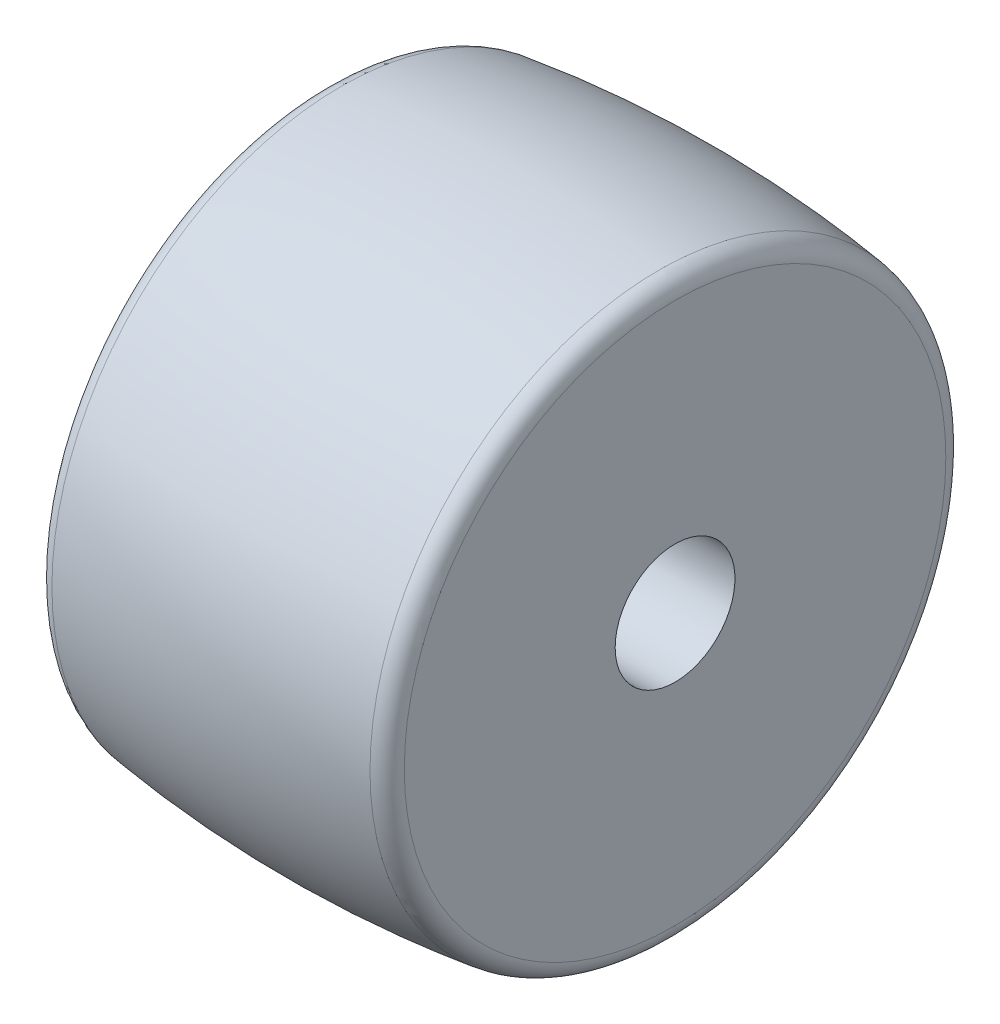
from build123d import *


with BuildPart() as part:
    # 草图1 → 旋转1 (revolve)
    with BuildSketch(Plane.XY, mode=Mode.PRIVATE) as revolve_1_sk:
        with BuildLine():
            Line((-19, 6.5), (19, 6.5))
            Line((19, 6.5), (19, 29.38798244))
            ThreePointArc((19, 29.38798244), (18.503508031, 30.706869699), (17.260536398, 31.370940026))
            ThreePointArc((17.260536398, 31.370940026), (0, 32.5), (-17.260536398, 31.370940026))
            ThreePointArc((-17.260536398, 31.370940026), (-18.503508031, 30.706869699), (-19, 29.38798244))
            Line((-19, 29.38798244), (-19, 6.5))
        make_face()
    revolve(revolve_1_sk.sketch.rotate(Axis((50, 0, 0), (-1, 0, 0)), 270), axis=Axis((50, 0, 0), (-1, 0, 0)))


solid = part.part
